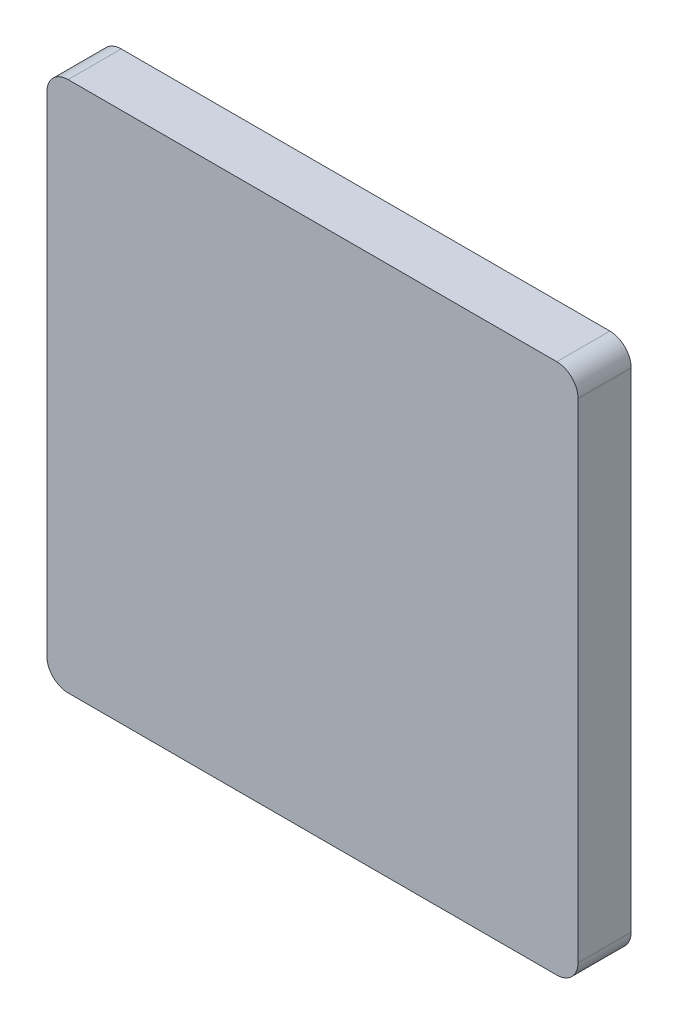
from build123d import *

# Parameters (mm, degrees)
SKETCH1_W           = 60
SKETCH1_H           = 60
SKETCH1_W_2         = 52
SKETCH1_H_2         = 52
BOSS_EXTRUDE1_DEPTH = 400
FILLET1_R           = 6
FILLET2_R           = 3
BOSS_EXTRUDE2_DEPTH = 5
CUT_EXTRUDE1_DEPTH  = 403.243707222


with BuildPart() as part:
    # Sketch1 → Boss-Extrude1 (new body)
    with BuildSketch(Plane.XY):
        Rectangle(SKETCH1_W, SKETCH1_H)
        Rectangle(SKETCH1_W_2, SKETCH1_H_2, mode=Mode.SUBTRACT)
    extrude(amount=BOSS_EXTRUDE1_DEPTH)

    # Fillet1
    fillet1_edges = [part.edges().sort_by_distance(p)[0] for p in [
        (30, -30, 200),
        (-30, -30, 200),
        (-30, 30, 200),
        (30, 30, 200),
    ]]
    fillet(fillet1_edges, radius=FILLET1_R)

    # Fillet2
    fillet2_edges = [part.edges().sort_by_distance(p)[0] for p in [
        (26, -26, 200),
        (26, 26, 200),
        (-26, 26, 200),
        (-26, -26, 200),
    ]]
    fillet(fillet2_edges, radius=FILLET2_R)

    # Sketch4 → Cut-Extrude1 (cut, through all)
    with BuildSketch(Plane(origin=(0, 0, 0), x_dir=(-1, 0, 0), z_dir=(0, 0, -1))):
        with BuildLine():
            Line((-30, 24), (-30, -24))
            ThreePointArc((-30, -24), (-28.242640687, -28.242640687), (-24, -30))
            Line((-24, -30), (24, -30))
            ThreePointArc((24, -30), (28.242640687, -28.242640687), (30, -24))
            Line((30, -24), (30, 24))
            ThreePointArc((30, 24), (28.242640687, 28.242640687), (24, 30))
            Line((24, 30), (-24, 30))
            ThreePointArc((-24, 30), (-28.242640687, 28.242640687), (-30, 24))
        make_face()
    extrude(amount=-CUT_EXTRUDE1_DEPTH, mode=Mode.SUBTRACT)


with BuildPart() as body_2:
    # Sketch2 → Boss-Extrude2 (new body)
    with BuildSketch(Plane(origin=(0, 0, 0), x_dir=(-1, 0, 0), z_dir=(0, 0, -1))):
        with BuildLine():
            Line((25, 23), (25, -23))
            ThreePointArc((25, -23), (24.414213562, -24.414213562), (23, -25))
            Line((23, -25), (-23, -25))
            ThreePointArc((-23, -25), (-24.414213562, -24.414213562), (-25, -23))
            Line((-25, -23), (-25, 23))
            ThreePointArc((-25, 23), (-24.414213562, 24.414213562), (-23, 25))
            Line((-23, 25), (23, 25))
            ThreePointArc((23, 25), (24.414213562, 24.414213562), (25, 23))
        make_face()
    extrude(amount=BOSS_EXTRUDE2_DEPTH)


solid = body_2.part
